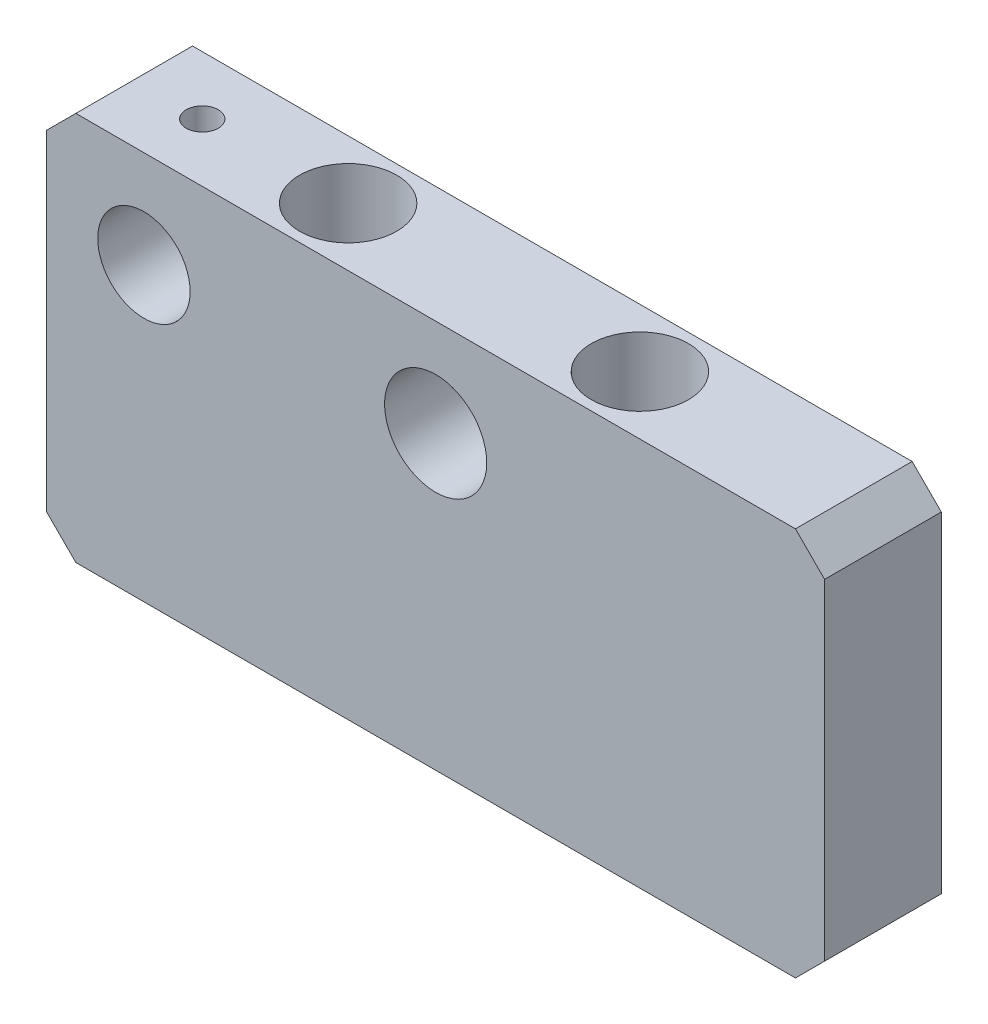
SolidWorks part; units mm, degrees
material "6061"
ref_plane "Front Plane" through (0, 0, 0) normal (0, 0, 1) x (1, 0, 0)
ref_plane "Top Plane" through (0, 0, 0) normal (0, 1, 0) x (1, 0, 0)
ref_plane "Right Plane" through (0, 0, 0) normal (1, 0, 0) x (0, 0, -1)
sketch "Sketch1" plane through (0, 0, 0) normal (0, 0, 1) x (1, 0, 0)
  line L1 (-40, 20) -> (40, 20)
  line L2 (-40, 20) -> (-40, -20)
  line L3 (-40, -20) -> (40, -20)
  line L4 (40, 20) -> (40, -20)
  line L5 (-40, 20) -> (40, -20) construction
  line L6 (-40, -20) -> (40, 20) construction
  point P0 (0, 0)
  dimension "D1" = 40
  dimension "D2" = 80
extrude "Boss-Extrude1" add sketch "Sketch1" along normal blind 12
sketch "Sketch2" plane through (0, 0, 12) normal (0, 0, 1) x (1, 0, 0)
  line L0 (0, 20) -> (0, -20) construction
  line L1 (40, 20) -> (-40, 20) construction
  line L2 (-40, -20) -> (40, -20) construction
  circle A0 centre (0, 10) radius 5.25
  circle A1 centre (-30, 10) radius 4.75
  dimension "D1" = 10.5
  dimension "D3" = 30
  dimension "D4" = 9.5
  dimension "D2" = 30
extrude "Cut-Extrude1" cut sketch "Sketch2" against normal through all
hole_wizard "CBORE for M5 Hex Socket Head Cap Screw1" positions "Sketch4" profile "Sketch3" counterbore size "M5" standard "Iso" end condition through all
sketch "Sketch4" plane through (0, 20, 0) normal (0, 1, 0) x (1, 0, 0)
  line L0 (0, 0) -> (0, -12) construction
  line L1 (40, -12) -> (-40, -12) construction
  line L4 (40, 0) -> (-40, 0) construction
  point P0 (-15, -6)
  point P2 (15, -6)
  dimension "D1" = 15
  dimension "D2" = 6
sketch "Sketch3" plane through (-15, 20, 6) normal (1, 0, 0) x (0, 0, 1)
  line L0 (0, 0) -> (0, 40)
  line L1 (0, 40) -> (2.75, 40)
  line L3 (2.75, 40) -> (2.75, 35)
  line L4 (2.75, 35) -> (5, 35)
  line L5 (5, 35) -> (5, 0)
  line L7 (5, 0) -> (0, 0)
  line L11 (0, -6.35) -> (0, 107.95) construction
  dimension "通孔孔直径" = 5.5
  dimension "通孔孔深度" = 40
  dimension "柱形沉头孔直径" = 10
  dimension "柱形沉头孔深度" = 35
chamfer "Chamfer1" distance 3 angle 45 4 edges at (-40, -20, 6) (40, -20, 6) (40, 20, 6) (-40, 20, 6)
hole_wizard "M4 Tapped Hole1" positions "Sketch6" profile "Sketch5" tap size "M4" standard "Iso"
sketch "Sketch6" plane through (0, 20, 0) normal (0, 1, 0) x (1, 0, 0)
  line L1 (37, 0) -> (-37, 0) construction
  line L2 (-40, -12) -> (-40, 0) construction
  point P0 (-30, -6)
  dimension "D1" = 6
  dimension "D2" = 10
sketch "Sketch5" plane through (-30, 20, 6) normal (1, 0, 0) x (0, 0, 1)
  line L0 (0, 0) -> (0, 11.0914)
  line L1 (0, 11.0914) -> (1.65, 10.1)
  line L2 (1.65, 10.1) -> (1.65, 0)
  line L5 (1.65, 0) -> (0, 0)
  line L10 (0, 11.0914) -> (-1.65, 10.1) construction
  line L11 (0, -6.35) -> (0, 107.95) construction
  dimension "螺纹孔钻头直径" = 3.3
  dimension "螺纹孔钻头深度" = 10.1
  dimension "导头角度" = 118
cosmetic thread "Hole thread1"
